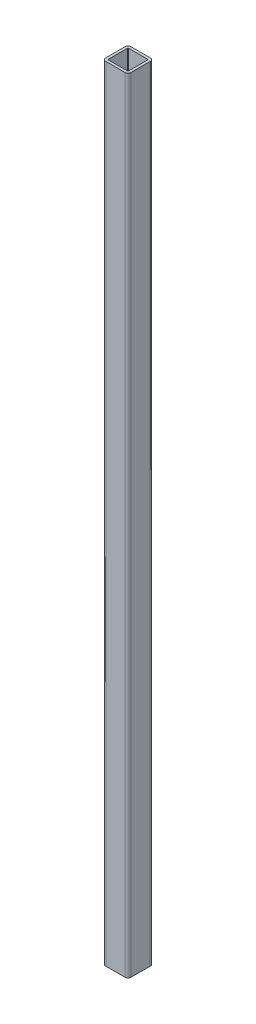
SolidWorks part; units mm, degrees
ref_plane "Front" through (0, 0, 0) normal (0, 0, 1) x (1, 0, 0)
ref_plane "Top" through (0, 0, 0) normal (0, 1, 0) x (1, 0, 0)
ref_plane "Right" through (0, 0, 0) normal (1, 0, 0) x (0, 0, -1)
sketch "草图1" plane through (0, 0, 0) normal (0, 1, 0) x (1, 0, 0)
  line L0 (-19, -7.2781) -> (19, -7.2781)
  line L1 (-19, -12.2781) -> (19, -12.2781)
  line L2 (-25, -6.2781) -> (-25, 31.7219)
  line L3 (-19, 37.7219) -> (19, 37.7219)
  line L4 (25, -6.2781) -> (25, 31.7219)
  line L5 (20, -6.2781) -> (20, 31.7219)
  line L6 (-19, 32.7219) -> (19, 32.7219)
  line L11 (-20, -6.2781) -> (-20, 31.7219)
  arc A0 (-19, -12.2781) -> (-25, -6.2781) centre (-19, -6.2781) cw
  arc A1 (19, -12.2781) -> (25, -6.2781) centre (19, -6.2781) ccw
  arc A2 (19, 37.7219) -> (25, 31.7219) centre (19, 31.7219) cw
  arc A3 (-25, 31.7219) -> (-19, 37.7219) centre (-19, 31.7219) cw
  arc A4 (19, -7.2781) -> (20, -6.2781) centre (19, -6.2781) ccw
  arc A5 (19, 32.7219) -> (20, 31.7219) centre (19, 31.7219) cw
  arc A6 (-20, 31.7219) -> (-19, 32.7219) centre (-19, 31.7219) cw
  arc A7 (-19, -7.2781) -> (-20, -6.2781) centre (-19, -6.2781) cw
  point P9 (25, -12.2781)
  point P12 (25, 37.7219)
  point P15 (-25, 37.7219)
  dimension "D3" = 6
  dimension "D1" = 50
  dimension "D2" = 50
  dimension "D4" = 5
extrude "凸台-拉伸1" add sketch "草图1" along normal blind 1550
